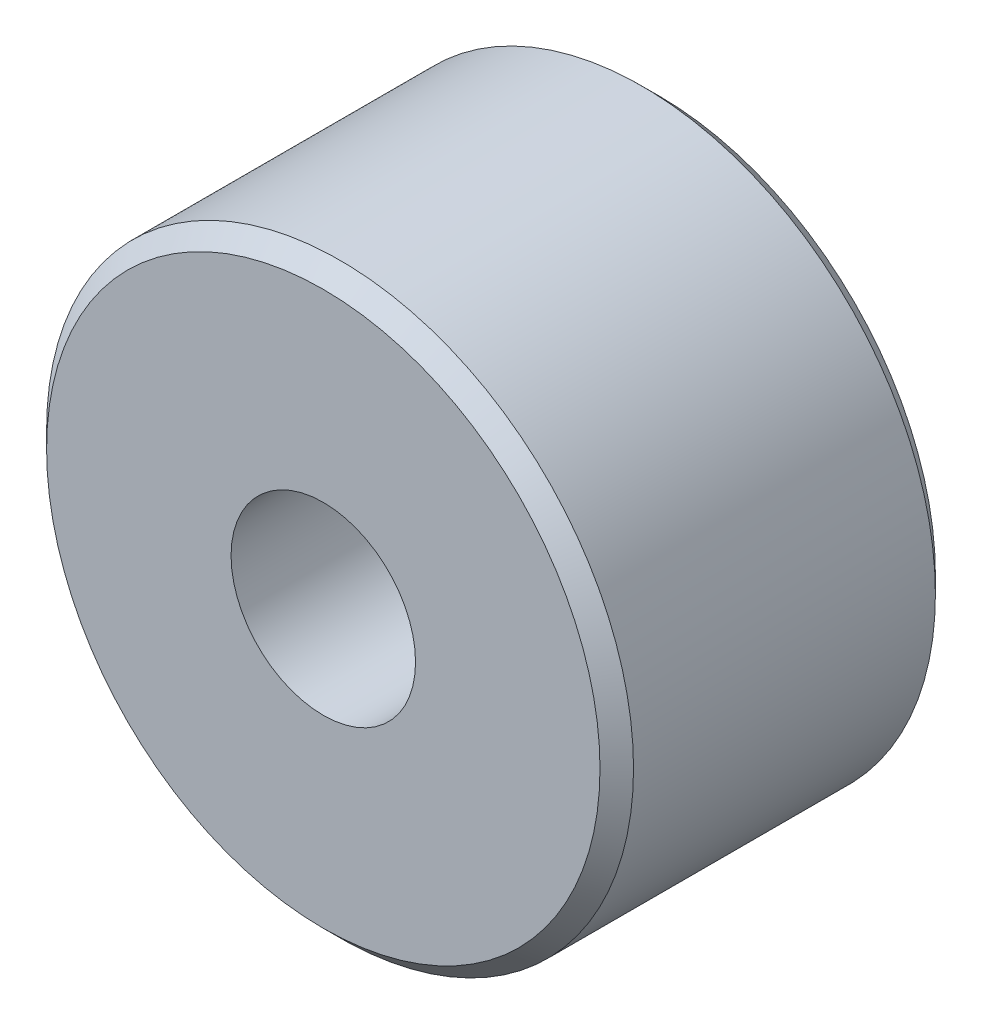
SolidWorks part; units mm, degrees
ref_plane "Front Plane" through (0, 0, 0) normal (0, 0, 1) x (1, 0, 0)
ref_plane "Top Plane" through (0, 0, 0) normal (0, 1, 0) x (1, 0, 0)
ref_plane "Right Plane" through (0, 0, 0) normal (1, 0, 0) x (0, 0, -1)
sketch "Sketch1" plane through (0, 0, 0) normal (0, 0, 1) x (1, 0, 0)
  circle A0 centre (0, 0) radius 8.75
  circle A1 centre (0, 0) radius 2.75
  dimension "D1" = 5.5
  dimension "D2" = 17.5
extrude "Boss-Extrude1" add sketch "Sketch1" along normal blind 10
sketch "Sketch2" plane through (0, 0, 0) normal (0, 0, -1) x (-1, 0, 0)
  circle A0 centre (0, 0) radius 5
  dimension "D1" = 10
extrude "Cut-Extrude1" cut sketch "Sketch2" against normal blind 5.5
chamfer "Chamfer1" distance 0.5 angle 45 2 edges at (8.75, 0, 0) (8.75, 0, 10)
